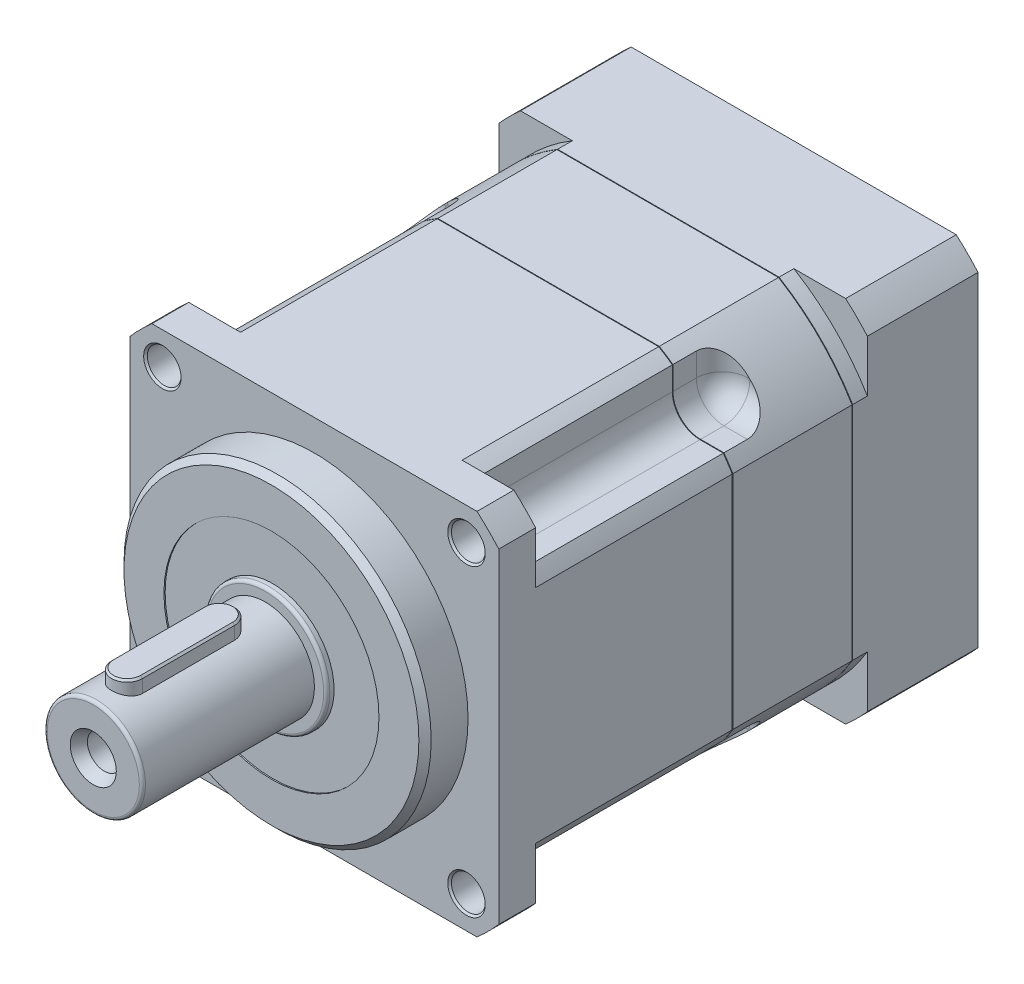
SolidWorks part; units mm, degrees
ref_plane "前视基准面" through (0, 0, 0) normal (0, 0, 1) x (1, 0, 0)
ref_plane "上视基准面" through (0, 0, 0) normal (0, 1, 0) x (1, 0, 0)
ref_plane "右视基准面" through (0, 0, 0) normal (1, 0, 0) x (0, 0, -1)
sketch "草图1" plane through (0, 0, 0) normal (0, 0, 1) x (1, 0, 0)
  line L1 (-26.4575, 30) -> (26.4575, 30)
  line L2 (-30, 26.4575) -> (-30, -26.4575)
  line L3 (-26.4575, -30) -> (26.4575, -30)
  line L4 (30, 26.4575) -> (30, -26.4575)
  arc A0 (-26.4575, 30) -> (-30, 26.4575) centre (0, 0) ccw
  arc A1 (-30, -26.4575) -> (-26.4575, -30) centre (0, 0) ccw
  arc A2 (26.4575, -30) -> (30, -26.4575) centre (0, 0) ccw
  arc A3 (30, 26.4575) -> (26.4575, 30) centre (0, 0) ccw
  dimension "D1" = 30
  dimension "D4" = 30
extrude "凸台-拉伸1" add sketch "草图1" along normal blind 6
sketch "草图2" plane through (0, 0, 6) normal (0, 0, 1) x (1, 0, 0)
  circle A0 centre (0, 0) radius 25
extrude "凸台-拉伸2" add sketch "草图2" along normal blind 7
sketch "草图3" plane through (0, 0, 0) normal (0, 0, -1) x (-1, 0, 0)
  line L1 (-18.0278, 30) -> (18.0278, 30)
  line L2 (-30, 18.0278) -> (-30, -18.0278)
  line L3 (-18.0278, -30) -> (18.0278, -30)
  line L4 (30, 18.0278) -> (30, -18.0278)
  arc A0 (-18.0278, 30) -> (-30, 18.0278) centre (0, 0) ccw
  arc A1 (-30, -18.0278) -> (-18.0278, -30) centre (0, 0) ccw
  arc A2 (18.0278, -30) -> (30, -18.0278) centre (0, 0) ccw
  arc A3 (30, 18.0278) -> (18.0278, 30) centre (0, 0) ccw
  dimension "D1" = 30
  dimension "D3" = 30
extrude "凸台-拉伸3" add sketch "草图3" along normal blind 32
sketch "草图4" plane through (0, 0, -32) normal (0, 0, -1) x (-1, 0, 0)
  line L1 (-34.1586, 33.3913) -> (-20.25, 33.3913)
  line L2 (-34.1586, 33.3913) -> (-34.1586, 20.25)
  line L3 (-34.1586, 20.25) -> (-20.25, 20.25)
  line L4 (-20.25, 33.3913) -> (-20.25, 20.25)
  dimension "D1" = 20.25
  dimension "D2" = 20.25
extrude "切除-拉伸1" cut sketch "草图4" against normal up to surface (32 mm away) up to face at (25.6924, 26.578, 0)
pattern_circular "阵列(圆周)1" count 4 over 360 about axis through (0, 0, 0) along (0, 0, 1) of "切除-拉伸1"
fillet "圆角1" radius 4.5 4 edges at (20.25, -20.25, -16) (-20.25, -20.25, -16) (-20.25, 20.25, -16) (20.25, 20.25, -16)
sketch "草图5" plane through (0, 0, 6) normal (0, 0, 1) x (1, 0, 0)
  line L0 (0, 0) -> (-28.2843, 28.2843) construction
  circle A0 centre (0, 0) radius 35 construction
  arc A1 (-26.4575, 30) -> (-30, 26.4575) centre (0, 0) ccw construction
  circle A2 centre (-24.7487, 24.7487) radius 2.75
extrude "切除-拉伸2" cut sketch "草图5" against normal blind 32
pattern_circular "阵列(圆周)2" count 4 over 360 about axis through (0, 0, 0) along (0, 0, 1) of "切除-拉伸2"
ref_plane "基准面1" through (0, 0, -32.1) normal (0, 0, -1) x (-1, 0, 0)
sketch "草图6" plane through (0, 0, -32.1) normal (0, 0, -1) x (-1, 0, 0)
  line L1 (-18.0278, 30) -> (18.0278, 30)
  line L2 (-30, 18.0278) -> (-30, -18.0278)
  line L3 (-18.0278, -30) -> (18.0278, -30)
  line L4 (30, 18.0278) -> (30, -18.0278)
  arc A0 (-18.0278, 30) -> (-30, 18.0278) centre (0, 0) ccw
  arc A1 (-30, -18.0278) -> (-18.0278, -30) centre (0, 0) ccw
  arc A2 (18.0278, -30) -> (30, -18.0278) centre (0, 0) ccw
  arc A3 (30, 18.0278) -> (18.0278, 30) centre (0, 0) ccw
  dimension "D1" = 30
  dimension "D3" = 30
extrude "凸台-拉伸4" add sketch "草图6" along normal blind 19.4 separate body
sketch "草图7" plane through (0, 0, -32.1) normal (0, 0, 1) x (1, 0, 0)
  line L1 (-36.173, 34.5423) -> (-20.25, 34.5423)
  line L2 (-36.173, 34.5423) -> (-36.173, 20.25)
  line L3 (-36.173, 20.25) -> (-20.25, 20.25)
  line L4 (-20.25, 34.5423) -> (-20.25, 20.25)
  dimension "D1" = 20.25
  dimension "D2" = 20.25
extrude "切除-拉伸3" cut sketch "草图7" against normal blind 8
pattern_circular "阵列(圆周)3" count 4 over 360 about axis through (0, 0, 0) along (0, 0, 1) of "切除-拉伸3"
fillet "圆角2" radius 4.5 4 edges at (-20.25, -20.25, -36.1) (20.25, -20.25, -36.1) (20.25, 20.25, -36.1) (-20.25, 20.25, -36.1)
fillet "圆角3" radius 4.2 12 edges at (20.25, 26.6486, -40.1) (26.6486, 20.25, -40.1) (-26.6486, 20.25, -40.1) (-20.25, 26.6486, -40.1) (-20.25, -26.6486, -40.1) (-26.6486, -20.25, -40.1) (26.6486, -20.25, -40.1) (20.25, -26.6486, -40.1) (21.568, 21.568, -40.1) (-21.568, 21.568, -40.1) (-21.568, -21.568, -40.1) (21.568, -21.568, -40.1)
chamfer "倒角1" distance 1 angle 45 1 edges at (25, 0, 13)
ref_plane "基准面2" through (0, 0, -51.6) normal (0, 0, -1) x (-1, 0, 0)
sketch "草图8" plane through (0, 0, -51.6) normal (0, 0, -1) x (-1, 0, 0)
  line L0 (18.0278, 30) -> (-18.0278, 30) construction
  line L1 (-30, 18.0278) -> (-30, -18.0278) construction
  line L2 (-18.0278, -30) -> (18.0278, -30) construction
  line L3 (30, -18.0278) -> (30, 18.0278) construction
  line L4 (18.0278, 30) -> (-18.0278, 30)
  line L5 (-30, 18.0278) -> (-30, -18.0278)
  line L6 (-18.0278, -30) -> (18.0278, -30)
  line L7 (30, -18.0278) -> (30, 18.0278)
  arc A0 (30, 18.0278) -> (18.0278, 30) centre (0, 0) ccw construction
  arc A1 (-18.0278, 30) -> (-30, 18.0278) centre (0, 0) ccw construction
  arc A2 (-30, -18.0278) -> (-18.0278, -30) centre (0, 0) ccw construction
  arc A3 (18.0278, -30) -> (30, -18.0278) centre (0, 0) ccw construction
  arc A4 (30, 18.0278) -> (18.0278, 30) centre (0, 0) ccw
  arc A5 (-18.0278, 30) -> (-30, 18.0278) centre (0, 0) ccw
  arc A6 (-30, -18.0278) -> (-18.0278, -30) centre (0, 0) ccw
  arc A7 (18.0278, -30) -> (30, -18.0278) centre (0, 0) ccw
extrude "凸台-拉伸5" add sketch "草图8" along normal blind 2.4 separate body
sketch "草图9" plane through (0, 0, -54) normal (0, 0, -1) x (-1, 0, 0)
  line L1 (-26.4575, 30) -> (26.4575, 30)
  line L2 (-30, 26.4575) -> (-30, -26.4575)
  line L3 (-26.4575, -30) -> (26.4575, -30)
  line L4 (30, 26.4575) -> (30, -26.4575)
  arc A0 (-26.4575, 30) -> (-30, 26.4575) centre (0, 0) ccw
  arc A1 (-30, -26.4575) -> (-26.4575, -30) centre (0, 0) ccw
  arc A2 (26.4575, -30) -> (30, -26.4575) centre (0, 0) ccw
  arc A3 (30, 26.4575) -> (26.4575, 30) centre (0, 0) ccw
  dimension "D1" = 30
  dimension "D3" = 30
extrude "凸台-拉伸6" add sketch "草图9" along normal blind 18
sketch "草图10" plane through (0, 0, -72) normal (0, 0, -1) x (-1, 0, 0)
  circle A0 centre (0, 0) radius 25
extrude "切除-拉伸4" cut sketch "草图10" against normal blind 5
sketch "草图11" plane through (0, 0, -72) normal (0, 0, -1) x (-1, 0, 0)
  line L0 (0, 0) -> (0, -25) construction
  line L1 (0, 0) -> (6.4705, -24.1481)
  circle A0 centre (0, 0) radius 25 construction
  circle A1 centre (6.4705, -24.1481) radius 4
  dimension "D1" = 15
extrude "切除-拉伸5" cut sketch "草图11" against normal blind 12 contours A1
pattern_circular "阵列(圆周)4" count 4 over 360 about axis through (0, 0, 0) along (0, 0, 1) of "切除-拉伸5"
sketch "草图12" plane through (0, 0, -72) normal (0, 0, -1) x (-1, 0, 0)
  line L0 (0, 0) -> (-24.1481, -6.4705) construction
  line L1 (0, 0) -> (-15.733, -19.4286) construction
  arc A0 (-22.8071, -10.239) -> (2.5363, -24.871) centre (0, 0) ccw construction
  circle A1 centre (-15.733, -19.4286) radius 4
  dimension "D1" = 36
extrude "切除-拉伸6" cut sketch "草图12" against normal blind 12
pattern_circular "阵列(圆周)5" count 2 over 360 about axis through (0, 0, 0) along (0, 0, 1) of "切除-拉伸6"
sketch "草图13" plane through (0, 0, -67) normal (0, 0, -1) x (-1, 0, 0)
  circle A0 centre (0, 0) radius 19
extrude "切除-拉伸7" cut sketch "草图13" against normal blind 13
sketch "草图14" plane through (0, 0, -60) normal (0, 0, -1) x (-1, 0, 0)
  line L1 (-5.6437, 25.789) -> (-7.4781, 25.6846)
  line L2 (-7.4781, 25.6846) -> (-8.3049, 24.0438)
  line L3 (-8.3049, 24.0438) -> (-7.2973, 22.5073)
  line L4 (-7.2973, 22.5073) -> (-5.4629, 22.6117)
  line L5 (-5.4629, 22.6117) -> (-4.6361, 24.2525)
  line L6 (-4.6361, 24.2525) -> (-5.6437, 25.789)
  circle A0 centre (-6.4705, 24.1481) radius 3
  circle A1 centre (-6.4705, 24.1481) radius 1.5912 construction
extrude "凸台-拉伸7" add sketch "草图14" along normal blind 6
pattern_circular "阵列(圆周)6" count 4 over 360 about axis through (0, 0, 0) along (0, 0, 1) of "凸台-拉伸7"
sketch "草图15" plane through (0, 0, -60) normal (0, 0, -1) x (-1, 0, 0)
  line L1 (-14.8157, -17.8764) -> (-16.6186, -17.8581)
  line L2 (-16.6186, -17.8581) -> (-17.5359, -19.4103)
  line L3 (-17.5359, -19.4103) -> (-16.6503, -20.9809)
  line L4 (-16.6503, -20.9809) -> (-14.8474, -20.9992)
  line L5 (-14.8474, -20.9992) -> (-13.9301, -19.447)
  line L6 (-13.9301, -19.447) -> (-14.8157, -17.8764)
  circle A0 centre (-15.733, -19.4286) radius 3
  circle A1 centre (-15.733, -19.4286) radius 1.5615 construction
extrude "凸台-拉伸8" add sketch "草图15" along normal blind 6
pattern_circular "阵列(圆周)7" count 2 over 360 about axis through (0, 0, 0) along (0, 0, 1) of "凸台-拉伸8"
sketch "草图16" plane through (0, 0, -72) normal (0, 0, -1) x (-1, 0, 0)
  line L0 (0, 0) -> (-24.7487, 24.7487)
  circle A0 centre (0, 0) radius 35
hole_wizard "M4 螺纹孔1" positions "3D草图1" profile "草图17" tap size "M4" standard "GB"
sketch3d "3D草图1"
  point P0 (24.7487, 24.7487, -72)
sketch "草图17" plane through (24.7487, 24.7487, -72) normal (1, 0, 0) x (0, 1, 0)
  line L0 (0, 0) -> (0, 16.4914)
  line L1 (0, 16.4914) -> (1.65, 15.5)
  line L2 (1.65, 15.5) -> (1.65, 0)
  line L5 (1.65, 0) -> (0, 0)
  line L10 (0, 16.4914) -> (-1.65, 15.5) construction
  line L11 (0, -6.35) -> (0, 107.95) construction
  dimension "螺纹孔钻头直径" = 3.3
  dimension "螺纹孔钻头深度" = 15.5
  dimension "导头角度" = 118
cosmetic thread "孔螺蚊线1" parameters "D1"=12, "D2"=4
pattern_circular "阵列(圆周)8" count 4 over 360 about axis through (0, 0, 0) along (0, 0, 1) of "M4 螺纹孔1"
sketch "草图18" plane through (0, 0, -54) normal (0, 0, -1) x (-1, 0, 0)
  circle A0 centre (0, 0) radius 16.5
extrude "凸台-拉伸9" add sketch "草图18" along normal blind 11.5
chamfer "倒角2" distance 1 angle 45 1 edges at (-16.5, 0, -65.5)
sketch "草图19" plane through (0, 0, -72) normal (0, 0, -1) x (-1, 0, 0)
  circle A0 centre (0, 0) radius 7
extrude "切除-拉伸8" cut sketch "草图19" against normal blind 34
sketch "草图20" plane through (0, 0, -65.5) normal (0, 0, -1) x (-1, 0, 0)
  line L1 (-17.4577, 0.5) -> (18.2251, 0.5)
  line L2 (-17.4577, 0.5) -> (-17.4577, -0.5)
  line L3 (-17.4577, -0.5) -> (18.2251, -0.5)
  line L4 (18.2251, 0.5) -> (18.2251, -0.5)
  dimension "D1" = 0.5
  dimension "D2" = 1
extrude "切除-拉伸9" cut sketch "草图20" against normal up to surface (11.5 mm away) up to face at (-19, 0, -54)
sketch "草图21" plane through (0, 0, 13) normal (0, 0, 1) x (1, 0, 0)
  circle A0 centre (0, 0) radius 8
extrude "凸台-拉伸10" add sketch "草图21" along normal blind 29
sketch "草图22" plane through (0, 0, 13) normal (0, 0, 1) x (1, 0, 0)
  circle A0 centre (0, 0) radius 10
extrude "凸台-拉伸11" add sketch "草图22" along normal blind 1
fillet "圆角4" radius 0.5 1 edges at (10, 0, 14)
fillet "圆角5" radius 0.5 1 edges at (8, 0, 42)
sketch "草图23" plane through (0, 0, 13) normal (0, 0, 1) x (1, 0, 0)
  circle A0 centre (0, 0) radius 17.5
  circle A1 centre (0, 0) radius 10
extrude "切除-拉伸10" cut sketch "草图23" against normal blind 0.2
sketch "草图24" plane through (0, 0, 0) normal (0, 1, 0) x (1, 0, 0)
  line L1 (-7.5, -42) -> (7.5, -42) construction
  line L2 (-2.5, -21.5) -> (-2.5, -36.5)
  line L3 (2.5, -21.5) -> (2.5, -36.5)
  arc A0 (-2.5, -36.5) -> (2.5, -36.5) centre (0, -36.5) ccw
  arc A1 (2.5, -21.5) -> (-2.5, -21.5) centre (0, -21.5) ccw
  dimension "D1" = 15
  dimension "D2" = 5.5
extrude "凸台-拉伸12" add sketch "草图24" along normal blind 10
chamfer "倒角3" distance 0.3 angle 45 8 edges at (-24.7487, -21.9987, 6) (21.9987, -24.7487, 6) (24.7487, 21.9987, 6) (-21.9987, 24.7487, 6) (-2.5, 10, 29) (0, 10, 39) (0, 10, 19) (2.5, 10, 29)
sketch "草图25" plane through (0, 0, 42) normal (0, 0, 1) x (1, 0, 0)
  circle A0 centre (0, 0) radius 2.75
extrude "切除-拉伸11" cut sketch "草图25" against normal blind 4.8
sketch "草图26" plane through (0, 0, 42) normal (0, 0, 1) x (1, 0, 0)
  circle A0 centre (0, 0) radius 3.75
ref_plane "基准面3" through (0, 0, 40.2) normal (0, 0, 1) x (1, 0, 0)
sketch "草图27" plane through (0, 0, 40.2) normal (0, 0, 1) x (1, 0, 0)
  circle A0 centre (0, 0) radius 2.75 construction
  circle A1 centre (0, 0) radius 2.75
loft "切除-放样1" cut profiles "草图26", "草图27"
hole_wizard "M5 螺纹孔1" positions "3D草图2" profile "草图28" tap size "M5" standard "GB"
sketch3d "3D草图2"
  line L0 (0, 0, 37.2) -> (0, 0, 40.2) construction
  point P0 (0, 0, 37.2)
sketch "草图28" plane through (0, 0, 37.2) normal (1, 0, 0) x (0, -1, 0)
  line L0 (0, 0) -> (0, 20.4618)
  line L1 (0, 20.4618) -> (2.1, 19.2)
  line L2 (2.1, 19.2) -> (2.1, 0)
  line L5 (2.1, 0) -> (0, 0)
  line L10 (0, 20.4618) -> (-2.1, 19.2) construction
  line L11 (0, -6.35) -> (0, 107.95) construction
  dimension "螺纹孔钻头直径" = 4.2
  dimension "螺纹孔钻头深度" = 19.2
  dimension "导头角度" = 118
cosmetic thread "孔螺蚊线2" parameters "D1"=15.2, "D2"=5
